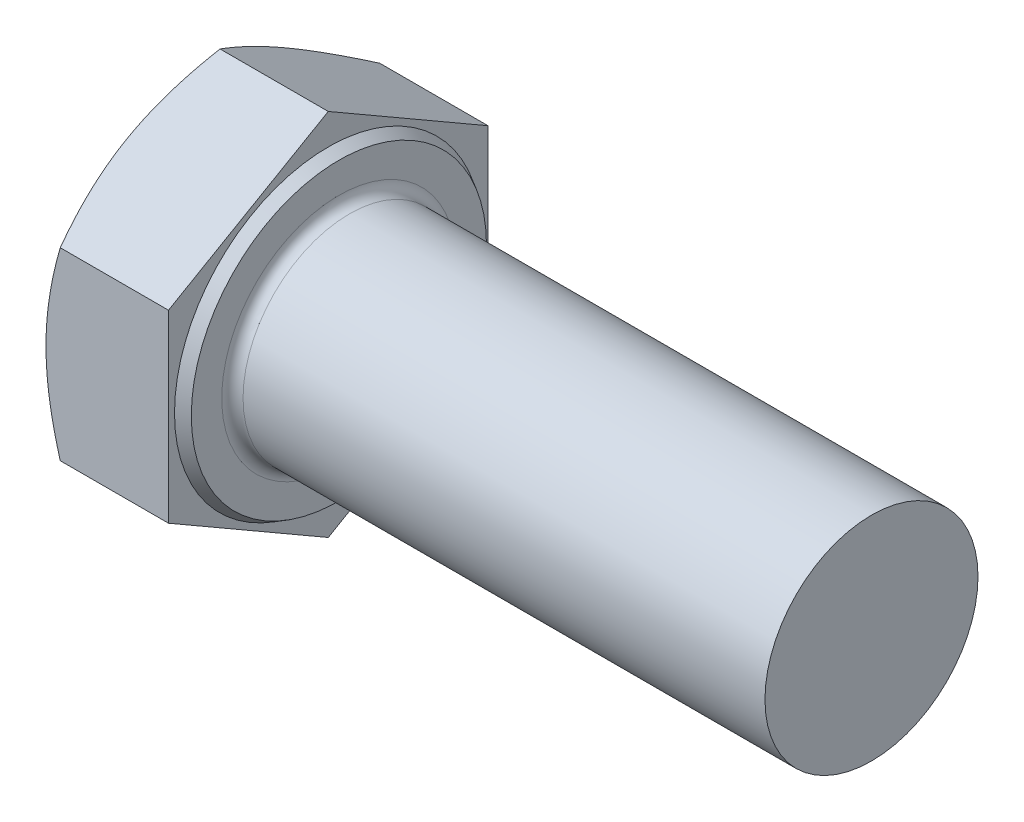
SolidWorks part; units mm, degrees
ref_plane "前视" through (0, 0, 0) normal (0, 0, 1) x (1, 0, 0)
ref_plane "上视" through (0, 0, 0) normal (0, 1, 0) x (1, 0, 0)
ref_plane "右视" through (0, 0, 0) normal (1, 0, 0) x (0, 0, -1)
sketch "草图1" plane through (0, 0, 0) normal (1, 0, 0) x (0, 0, -1)
  line L0 (9, 5.1962) -> (9, -5.1962)
  line L1 (-9, 5.1962) -> (-9, -5.1962)
  line L2 (9, -5.1962) -> (0, -10.3923)
  line L3 (0, -10.3923) -> (-9, -5.1962)
  line L4 (9, 5.1962) -> (0, 10.3923)
  line L5 (0, 10.3923) -> (-9, 5.1962)
  circle A0 centre (0, 0) radius 10.015 construction
  dimension "e" = 20.03
  dimension "s" = 18
  dimension "D2" = 120
  dimension "D3" = 9
  dimension "D4" = 9
  dimension "D5" = 9
extrude "基体-拉伸" add sketch "草图1" along normal blind 7.5
sketch "草图2" plane through (0, 0, 0) normal (0, 0, 1) x (1, 0, 0)
  line L0 (0, 5.1962) -> (0, -5.1962) construction
  line L1 (0, 0) -> (37.5, 0)
  line L2 (0, 0) -> (0, 6)
  line L3 (0, 6) -> (7.5, 6)
  line L4 (37.5, 0) -> (37.5, 4.4845)
  line L5 (7.5, 10.3923) -> (7.5, 5.1962) construction
  line L7 (0, 0) -> (49.5, 0) construction
  line L8 (37.5, -4.4845) -> (7.5, -6) construction
  line L9 (0, -6) -> (7.5, -6) construction
  line L10 (9.25, 6) -> (9.25, 0) construction
  line L11 (7.5, 15.24) -> (7.5, -1.27) construction
  line L12 (7.5, 5.1962) -> (7.5, -5.1962) construction
  line L13 (7.5, 6) -> (37.5, 6)
  line L14 (37.5, 6) -> (37.5, 4.4845)
  dimension "l" = 30
  dimension "d" = 12
  dimension "Minor_dia" = 8.969
  dimension "p" = 1.75
  dimension "b" = 30
  dimension "ds" = 12
revolve "凸台-旋转1" add sketch "草图2" angle 360 about L7
cosmetic thread "螺旋线1" parameters "Thread_length"=30, "Thread_minor"=8.969
sketch "草图3" plane through (0, 0, 0) normal (0, 0, 1) x (1, 0, 0)
  line L0 (0, 9) -> (3.6906, 15.3923)
  line L1 (0, 10.3923) -> (0, 5.1962) construction
  line L2 (3.6906, 15.3923) -> (3.6906, 20.3923)
  line L3 (3.6906, 20.3923) -> (-10, 20.3923)
  line L4 (-10, 20.3923) -> (-10, 9)
  line L5 (-10, 9) -> (0, 9)
  line L6 (0, 0) -> (99.06, 0) construction
  line L7 (7.5, 10.3923) -> (0, 10.3923) construction
  dimension "D1" = 9
  dimension "D2" = 5
  dimension "D3" = 10
  dimension "D4" = 5
  dimension "Head_ch_ang" = 30
revolve "切除-旋转1" cut sketch "草图3" angle 360 about L6
sketch "草图4" plane through (0, 0, 0) normal (0, 0, 1) x (1, 0, 0)
  line L0 (7.5, 0) -> (7.5, 8.315) construction
  line L2 (7.5, -6) -> (7.5, 6) construction
  line L3 (7.5, 10.3923) -> (7.5, 5.1962) construction
  line L4 (7.5, 8.315) -> (6.9, 8.6614)
  line L5 (0, 0) -> (95.25, 0) construction
  line L6 (0, 0) -> (49.5, 0) construction
  line L9 (6.9, 8.6614) -> (6.9, 10.3923)
  line L10 (7.5, 10.3923) -> (0.8038, 10.3923) construction
  line L11 (6.9, 10.3923) -> (7.5, 10.3923)
  line L12 (7.5, 10.3923) -> (7.5, 8.315)
  dimension "D1" = 120
  dimension "c" = 0.6
  dimension "dw" = 16.63
revolve "切除-旋转3" cut sketch "草图4" angle 360 about L5
fillet "圆角" radius 0.6 1 edges at (7.5, 0, -6)
sketch "草图6" plane through (0, 0, 0) normal (0, 0, 1) x (1, 0, 0)
  line L0 (0, 0) -> (37.5, 0) construction
  line L1 (37.5, -6) -> (37.5, 6) construction
  line L2 (37.5, 0) -> (37.5, 6) construction
  line L4 (36.625, 6) -> (38.375, 6)
  line L5 (36.625, 6) -> (37.5, 4.4845)
  line L6 (37.5, 4.4845) -> (38.375, 6)
  dimension "D1" = 1.75
revolve "切除-旋转4" [suppressed] cut sketch "草图6" angle 360 about L0
pattern_linear "阵列(线性)1" [suppressed]
